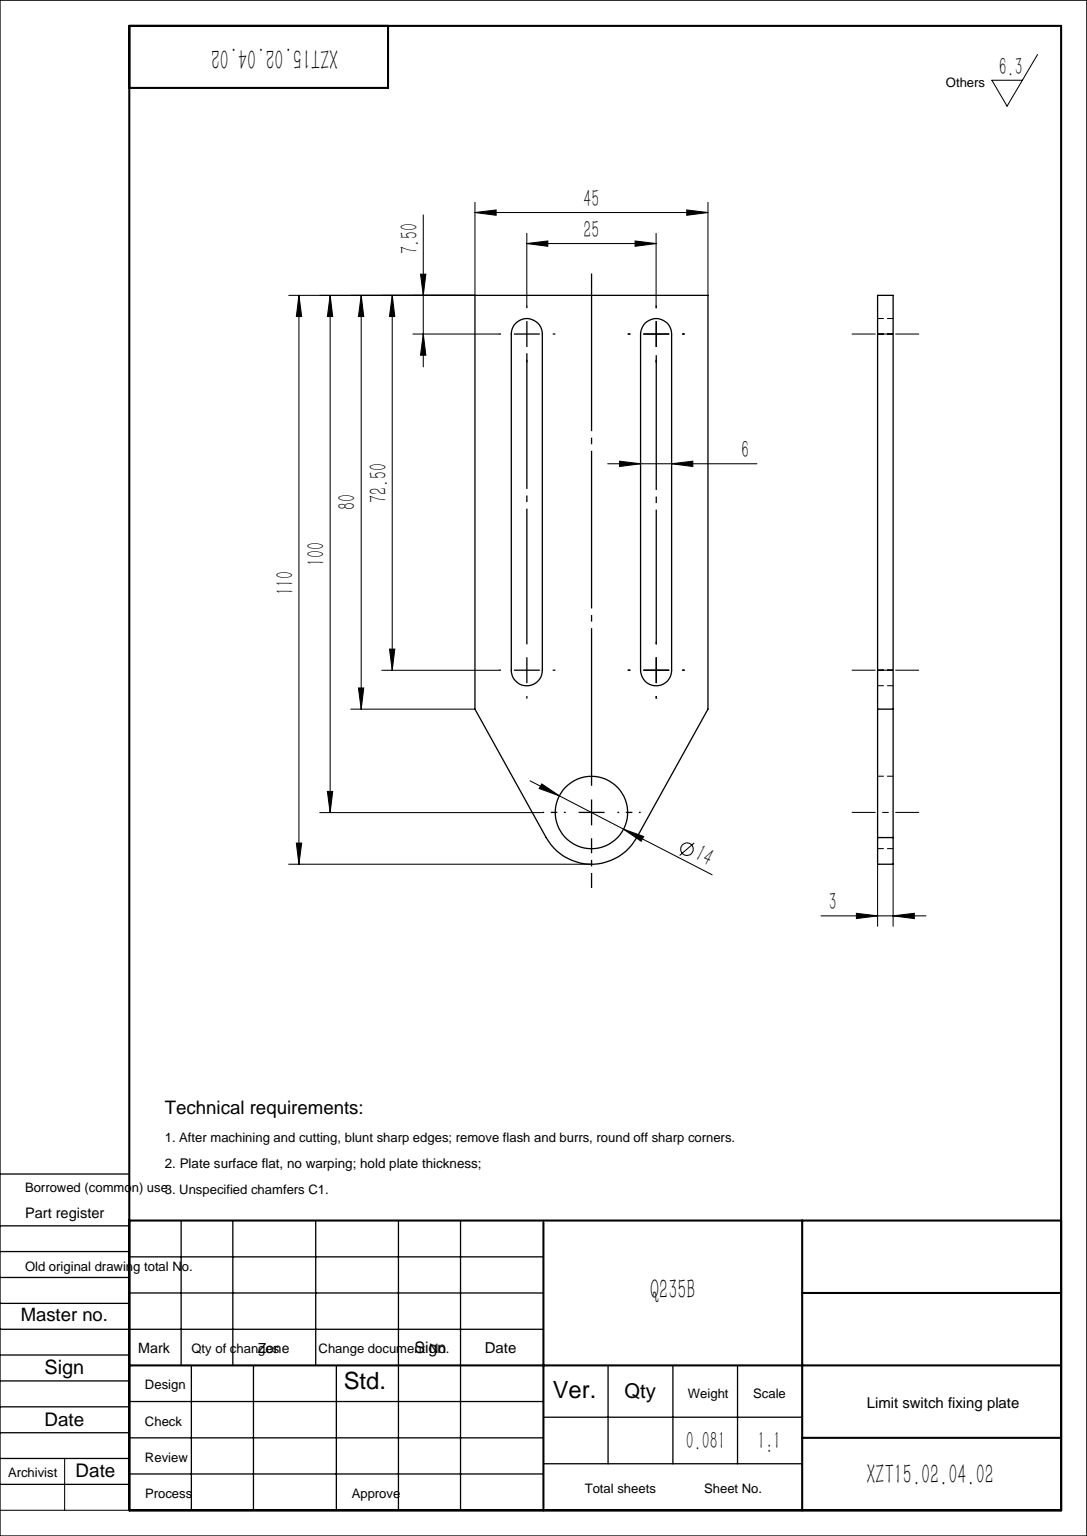
SolidWorks part; units mm, degrees
material "Q235B"
ref_plane "Front Plane" through (0, 0, 0) normal (0, 0, 1) x (1, 0, 0)
ref_plane "Top Plane" through (0, 0, 0) normal (0, 1, 0) x (1, 0, 0)
ref_plane "Right Plane" through (0, 0, 0) normal (1, 0, 0) x (0, 0, -1)
sketch "Sketch1" plane through (0, 0, 0) normal (0, 1, 0) x (1, 0, 0)
  line L0 (0, 0) -> (0, 100) construction
  line L1 (-22.5, 100) -> (22.5, 100)
  line L2 (22.5, 100) -> (22.5, 20)
  line L3 (22.5, 20) -> (8.7491, -4.8428)
  line L4 (-22.5, 20) -> (-8.7491, -4.8428)
  line L5 (-22.5, 100) -> (-22.5, 20)
  line L6 (-12.5, 27.5) -> (-12.5, 92.5) construction
  line L7 (-15.5, 27.5) -> (-15.5, 92.5)
  line L8 (-9.5, 27.5) -> (-9.5, 92.5)
  line L9 (12.5, 27.5) -> (12.5, 92.5) construction
  line L10 (15.5, 27.5) -> (15.5, 92.5)
  line L11 (9.5, 27.5) -> (9.5, 92.5)
  arc A0 (8.7491, -4.8428) -> (-8.7491, -4.8428) centre (0, 0) cw
  circle A1 centre (0, 0) radius 7
  arc A2 (-15.5, 27.5) -> (-9.5, 27.5) centre (-12.5, 27.5) ccw
  arc A3 (-9.5, 92.5) -> (-15.5, 92.5) centre (-12.5, 92.5) ccw
  arc A4 (15.5, 27.5) -> (9.5, 27.5) centre (12.5, 27.5) cw
  arc A5 (9.5, 92.5) -> (15.5, 92.5) centre (12.5, 92.5) cw
  point P7 (-12.5, 60)
  point P20 (12.5, 60)
  dimension "D1" = 45
  dimension "D2" = 110
  dimension "D4" = 14
  dimension "D5" = 65
  dimension "D3" = 100
  dimension "D6" = 7.5
  dimension "D7" = 12.5
  dimension "D8" = 6
  dimension "D9" = 80
extrude "Boss-Extrude1" add sketch "Sketch1" along normal blind 3
